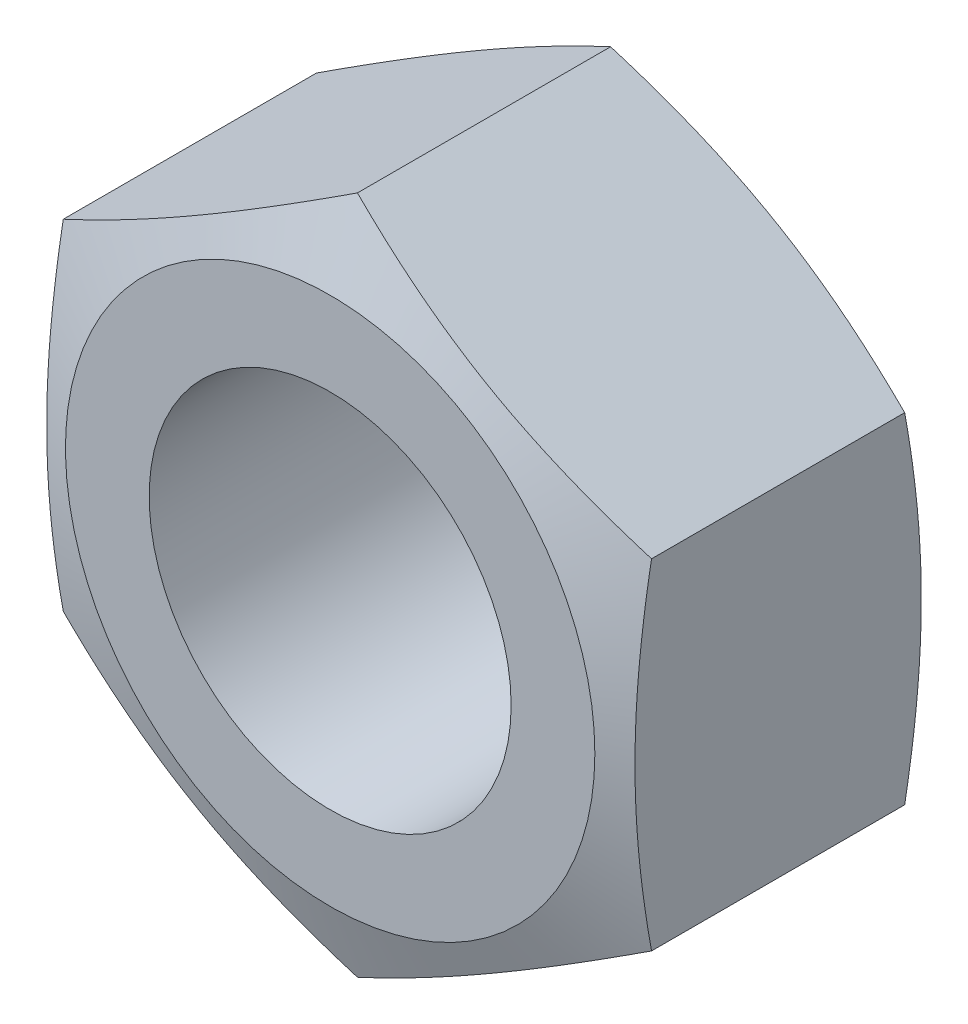
from build123d import *

# Parameters (mm, degrees)
EXTRUDE_1_DEPTH     = 6.8
SKETCH_5_R          = 4
CUT_EXTRUDE_1_DEPTH = 13.03425666


with BuildPart() as part:
    # 草图1 → 凸台-拉伸1 (new body)
    with BuildSketch(Plane.XY):
        Polygon((0, 7.505553499), (-6.5, 3.75277675), (-6.5, -3.75277675), (0, -7.505553499), (6.5, -3.75277675), (6.5, 3.75277675), align=None)
    extrude(amount=EXTRUDE_1_DEPTH)

    # 草图4 → 切除-旋转1 (revolve, cut)
    with BuildSketch(Plane(origin=(0, 0, 0), x_dir=(0, 0, -1), z_dir=(1, 0, 0)), mode=Mode.PRIVATE) as cut_revolve_1_sk:
        Polygon((-6.8, -5.85), (-6.197427805, -7.505553499), (-6.8, -7.505553499), align=None)
    cut_revolve_1 = revolve(cut_revolve_1_sk.sketch.rotate(Axis((0, 0, 6.8), (0, 0, -1)), 119.999999984), axis=Axis((0, 0, 6.8), (0, 0, -1)), mode=Mode.SUBTRACT)

    # 镜向1: 切除-旋转1 across plane
    add(cut_revolve_1.mirror(Plane.XY.offset(3.4)), mode=Mode.SUBTRACT)

    # 草图5 → 切除-拉伸1 (cut, through all)
    with BuildSketch(Plane.XY.offset(6.8)):
        Circle(SKETCH_5_R)
    extrude(amount=-CUT_EXTRUDE_1_DEPTH, mode=Mode.SUBTRACT)


solid = part.part
